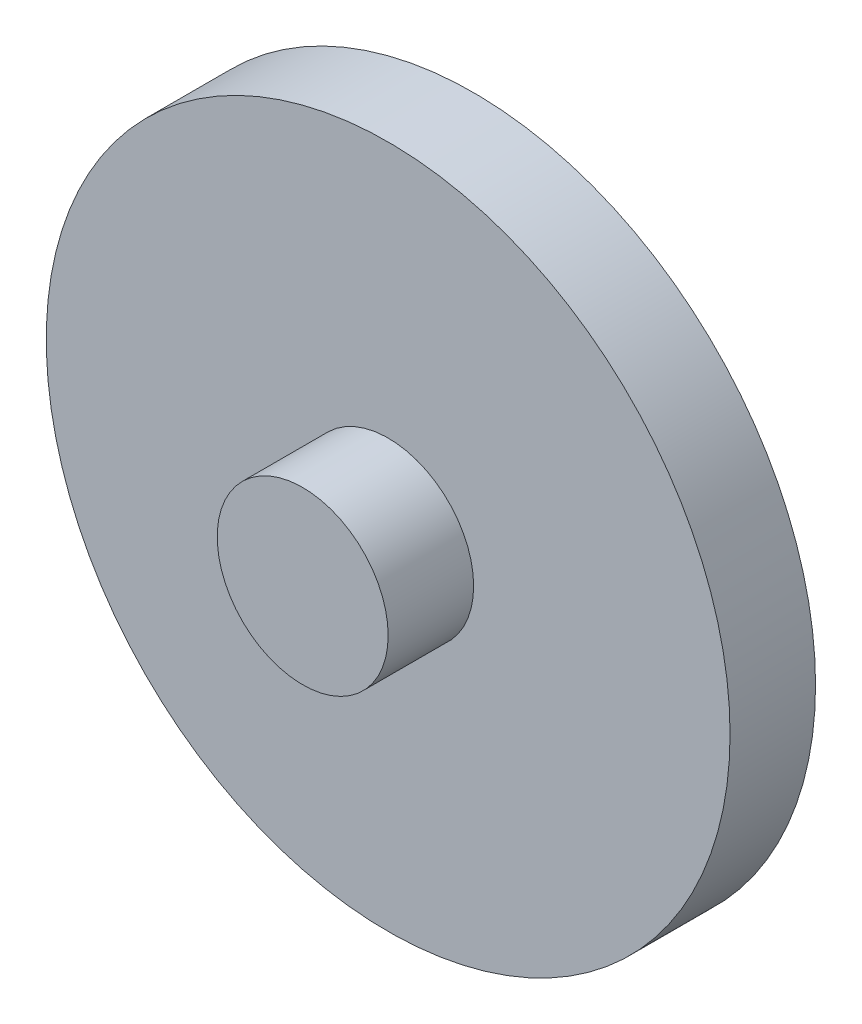
SolidWorks part; units mm, degrees
ref_plane "前视基准面" through (0, 0, 0) normal (0, 0, 1) x (1, 0, 0)
ref_plane "上视基准面" through (0, 0, 0) normal (0, 1, 0) x (1, 0, 0)
ref_plane "右视基准面" through (0, 0, 0) normal (1, 0, 0) x (0, 0, -1)
other "Configuration Table"
sketch "草图1" plane through (0, 0, 0) normal (0, 0, 1) x (1, 0, 0)
  circle A0 centre (0, 0) radius 40
  point P0 (0, 0)
  dimension "D1" = 80
extrude "凸台-拉伸1" add sketch "草图1" along normal blind 10
sketch "草图2" plane through (0, 0, 0) normal (0, 0, 1) x (1, 0, 0)
  circle A0 centre (0, 0) radius 10
  point P0 (0, 0)
  dimension "D1" = 20
extrude "凸台-拉伸2" add sketch "草图2" along normal blind 20
